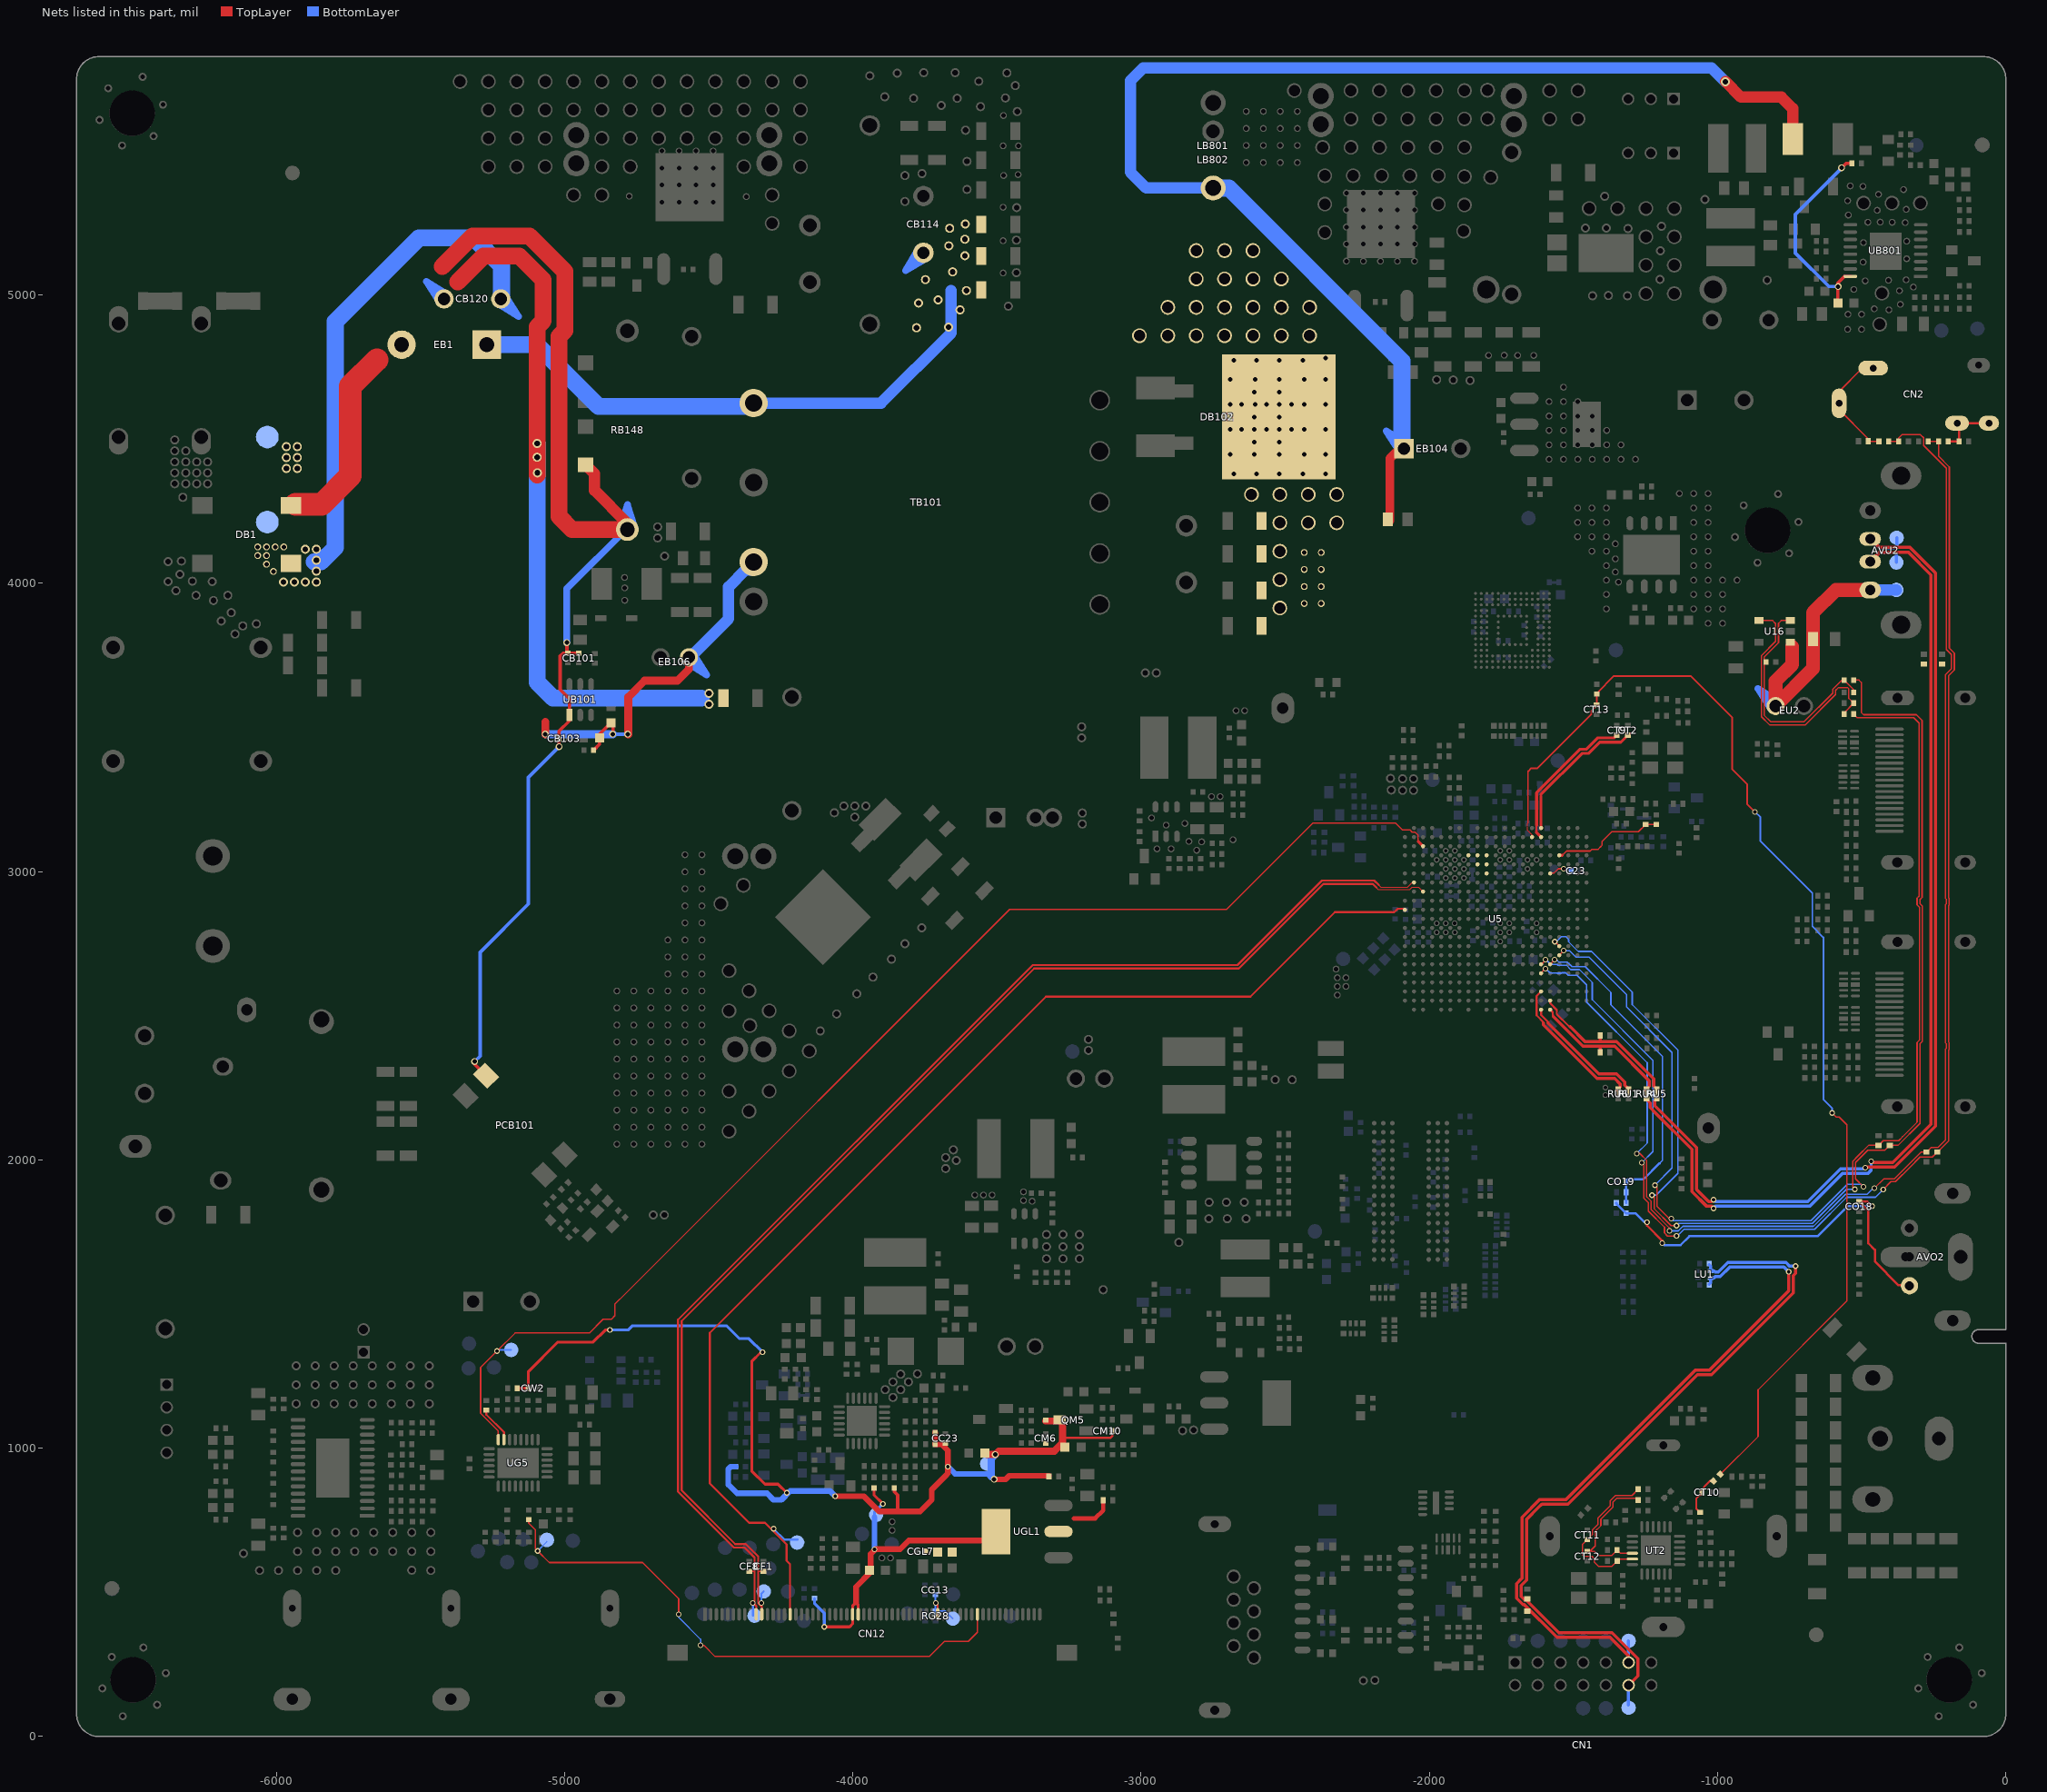
[diagram p0: the nets of this part, all layers, seen from the top]
# Altium PCB MISC84395.PcbDoc (part 23 of 26)
Units mil, origin at the board's own origin, x right, y up, seen from the top; angles counter-clockwise.
Board outline 6692.91 x 5826.77 mil, 2 copper layers (TopLayer, BottomLayer), stack 61.855 mil thick; 951 components, 565 nets, 4374 pads, 1804 vias.
Unrouted connection lines stored in the file: 1.

## Via types
v1: diameter 19.68, hole 11.81, TopLayer to BottomLayer, tented both sides, 1262 vias
v2: diameter 23.62, hole 15.75, TopLayer to BottomLayer, tented both sides, 524 vias
v3: diameter 31.5, hole 19.68, TopLayer to BottomLayer, tented both sides, 11 vias
v4: diameter 24, hole 16, TopLayer to BottomLayer, tented both sides, 6 vias
v5: diameter 19, hole 11.81, TopLayer to BottomLayer, tented both sides, 1 vias

## Nets (pads, with @x,y where several pads share a name; then routed paths per layer and width w, separated by ;. In a path a pad name is that pad's centre, name@x,y a point inside that pad or via, vN(x,y) a via of type N, cw(c..) or ccw(c..) an arc to the next point about the centre after c; other vN are vias at no path point) (continued)
RXO4P/MLV1P: CN12.16 MLV1P.1 U5.M21 | length 4248.8
  TopLayer w3.94: U5.M21@-2088.96,2867.58 U5.M21@-2084.93,2867.58
  TopLayer w7: CN12.16@-4217.44,423.98 -4217.66,424.2 -4217.66,597.66 -4229.66,609.66 -4229.66,666.66 -4304.63,741.63 -4359.87,741.63 -4496,877.76 -4496,1400.29 -3330.29,2566 -2620.46,2566 -2327.36,2859.1 -2236.83,2859.1 -2121.75,2859.1 -2109.53,2871.33 -2088.68,2871.33 U5.M21@-2084.93,2867.58
  BottomLayer w7: v1(-4275,721) -4237,683 MLV1P.1@-4192,683
RXOCN/MLVCKN: CF8.2 CN12.10 MLVCKN.1 U5.R20 | length 4421.4
  TopLayer w3.94: -2175.77,2953.61 -2168.48,2946.32 -2075.73,2946.32 -2059.98,2962.07 U5.R20@-2053.43,2962.07
  TopLayer w7: CF8.2@-4359,573.11 -4340.66,573.11 ; v1(-4347,463) -4344.97,463 v1@-4340.55,458.58 ; CN12.10@-4335.55,423.98 -4334.49,425.05 -4334.49,452.51 v1@-4340.55,458.58 ; -2175.77,2953.61 -2191.26,2969.1 -2372.92,2969.1 -2666.02,2676 -3375.86,2676 -4606,1445.86 -4606,849.17 -4412.46,655.63 -4375.63,655.63 -4340.55,620.55 v1@-4340.55,458.58
  BottomLayer w7: MLVCKN.1@-4346,419 v1@-4346,458
RXOCP/MLVCKP: CF1.2 CN12.11 MLVCKP.1 U5.P19 | length 4443.9
  TopLayer w3.94: -2184.26,2945.13 -2177.58,2938.45 -2067.7,2938.45 -2059.83,2946.32 -2037.68,2946.32 U5.P19@-2021.94,2930.57
  TopLayer w7: -4327.81,573.26 CF1.2@-4310,573.26 ; v1(-4317,463) -4317,452 ; CN12.11@-4315.86,423.98 -4315.86,450.86 -4317,452 ; -2184.26,2945.13 -2196.23,2957.1 -2367.95,2957.1 -2661.05,2664 -3370.89,2664 -4594,1440.89 -4594,854.14 -4407.49,667.63 -4370.66,667.63 -4328.55,625.52 -4328.55,463.55 -4317,452
  BottomLayer w7: v1(-4317,463) -4317,495.5 MLVCKP.1@-4309.04,503.47
SD_CLK_IC: U5.U12
SD_CMD_IC: U5.V12
SD_D0_IC: U5.U13
SD_D1_IC: U5.T12
SD_D2_IC: U5.V13
SD_D3_IC: U5.V14
SET1: RG4.2 UG5.7 | length 127.7
  TopLayer w7: RG4.2@-5271,1132.27 -5271,1116.56 -5210.21,1055.77 UG5.7@-5210.21,1029.71
SGND: CB101.2 CB102.2 CB103.2 CB111.1 CB120.1 DB1.4 DB110.K EB1.2 EB106.2 pad.VIA5@-4499,3580 pad.VIA5@-4499,3618 pad.VIA5@-5094,4383 pad.VIA5@-5095.08,4437 pad.VIA5@-5095.08,4485 pad.VIA5@-5927,4398 pad.VIA5@-5927,4436 pad.VIA5@-5927,4474 pad.VIA5@-5965,4398 pad.VIA5@-5965,4436 pad.VIA5@-5965,4474 PCB101.3 RB103.1 RB104.1 RB130.1 RB148.1 TB101.5 TP-TDT.2 UB101.1 | length 8667.9
  TopLayer w11.81: v2(-5312,2341) -5312,2332 PCB101.3@-5272,2292 ; v2(-5018.49,3433.3) -5018.95,3433.76 CB103.2@-5018.95,3461.3 -5018.95,3486.83 -4982.89,3522.9 UB101.1@-4982.89,3543 -4982.89,3598.7 -5015.49,3631.3 -5015.49,3747.3 -5005.24,3757.55 RB103.1@-4988.43,3757.55 ; v2(-4991.77,3794.3) -4991.77,3760.89 RB103.1@-4988.43,3757.55 ; CB101.2@-4950.43,3757.55 RB103.1@-4988.43,3757.55 ; RB104.1@-4899.02,3421.3 -4878.68,3441.65 CB111.1@-4878.68,3464.3 -4878.68,3476.11 CB102.2@-4838.49,3516.3 -4831.49,3509.3 -4831.49,3477.3 v2(-4832.49,3476.3)
  TopLayer w27.56: v2(-5066.7,3476.3) -5066.7,3518.7 ; v2@-4778.8,3476.3 -4778.8,3605.2 -4722,3662 -4608,3662 -4568.57,3701.43 EB106.2@-4568.57,3743
  TopLayer w39.37: DB110.K@-4927,4410.85 -4896,4379.85 -4896,4322 -4782,4208 RB148.1@-4782,4186.25
  TopLayer w59.06: -5424.5,5098.5 -5319,5204 -5122,5204 -4999,5081 ; -5371,5045 -5281,5135 -5157,5135 -5074,5052 -5074,4910 -5095.08,4888.92 pad.VIA5@-5095.08,4375 ; -5043.89,5126 -4999,5081.11 -4999,5081 ; RB148.1@-4782,4186.25 -4974.25,4186.25 -5019.49,4231.49 -5019.49,4855.51 -4999,4876 -4999,5081
  TopLayer w78.74: DB1.4@-5933.21,4273 -5842.99,4273 -5742.99,4373 -5742.99,4683.01 -5651,4775
  BottomLayer w11.81: v2(-5312,2341) -5293,2360 -5293,2719.57 -5125.22,2887.35 -5125.22,3326.57 v2(-5018.49,3433.3) ; v2(-4832.49,3476.3) v2(-4780.49,3476.3)
  BottomLayer w23.62: v2(-4991.77,3794.3) -4991.77,3981.04 RB148.1@-4782,4190.81
  BottomLayer w27.56: v2(-5066.7,3476.3) v2(-4832.49,3476.3)
  BottomLayer w39.37: EB106.2@-4566.57,3741 -4431,3876.57 -4431,3987.13 -4371.87,4046.26 TB101.5@-4344.32,4046.26
  BottomLayer w59.06: pad.VIA5@-5095.08,4485 -5095.08,3657 -5039.38,3601.3 -4526,3601.3
SPDIF_OUT: AVO2.1 CO18.1 RO4.2 RO45.2 | length 1412
  TopLayer w8: v1(-1245,1784) -1245,1772.56 v1@-1192,1719.56 ; v1@-464.57,1838 -481.56,1855 CO18.1@-508.99,1855 -477.02,1823.03 -477.02,1710.56 -454.72,1688.26 -454.72,1647.72 -372.42,1565.42 AVO2.1@-348.43,1565.42
  BottomLayer w8: RO45.2@-1351.46,1851.06 -1351.46,1848.52 RO4.2@-1318,1815.06 -1284.7,1815.06 v1@-1253.65,1784 ; v1@-1185.29,1704.29 -1129.15,1704.29 -1098.28,1735.16 -653.4,1735.16 -549.12,1839.44 -465.13,1839.44 v1(-464.57,1840)
  other v1: -1192,1711
SPDIF_OUT_IC: CO19.2 DO1.K RO45.1 U5.F5 | length 1153.3
  TopLayer w5: U5.F5@-1580.99,2678.6 v1@-1565.65,2693.95
  BottomLayer w5: v1@-1565.75,2694.33 -1566.45,2695.03 -1559.99,2695.03 -1550.36,2685.4 -1520.83,2685.4 -1505.44,2670.01 -1459.39,2670.01 -1370.3,2580.92 -1370.3,2537.78 -1191.3,2358.78 -1191.3,1998.31 -1201.62,1988
  BottomLayer w8: RO45.1@-1318,1851.06 -1317.07,1851.99 DO1.K@-1317.07,1888 ; DO1.K@-1318,1888.93 CO19.2@-1318,1925.06 -1311.06,1932 -1257.62,1932 -1201.62,1988
  other v1: -1565.49,2694.59
STV: CN12.49 RG81.1 STV.1 | length 1984.8
  TopLayer w5: RG81.1@-5124,752.27 -5124,740 -5101.6,717.6 -5101.6,652.34 v1(-5093.26,644) -5052.76,603.5 -4729.22,603.5 -4604,478.28 v1(-4604,424) ; v1(-4528,316.5) -4516.94,316.5 -4477.94,277.5 -3735.11,277.5 -3682.37,330.24 -3599.58,330.24 -3567.83,361.99 CN12.49@-3567.83,418.08
  BottomLayer w5: v1(-5093.26,644) STV.1@-5061.26,676 ; v1(-4604,424) -4604,413.53 -4528,337.53 v1(-4528,316.5)
STV_IN: STV_IN.1 U5.W19 UG5.8 | length 4440.9
  TopLayer w5: UG5.8@-5229.9,1029.71 -5229.9,1059.9 -5291,1121 -5291,1280 v1(-5234.27,1336.73) -5171.5,1399.5 -4914.01,1399.5 -4866.01,1447.5 -4837.5,1447.5 -4825,1460 -4825,1499.8 -4786.59,1538.21 -3455.8,2869 -2703.54,2869 -2403.72,3168.82 -2118.04,3168.82 -2093.35,3144.14 -2067.15,3144.14 -2059.47,3136.46 -2049.71,3136.46 -2038.85,3125.59 -2038.85,3104.96
  TopLayer w10: -2038.85,3104.96 U5.W19@-2021.94,3088.05
  BottomLayer w5: v1@-5230,1341 STV_IN.1@-5185,1341
SYSTEM_RST_IC: R3.2 R21.1 U5.V4 | length 391.5
  TopLayer w5: U5.V4@-1548.31,3057.74 U5.V4@-1549.5,3056.56 U5.V4@-1546.22,3056.56 ; -1538.63,3057.74 -1537.44,3057.74 -1524.04,3071.14 -1441.86,3071.14 -1435.66,3077.34 -1414.8,3077.34 -1414.76,3077.38 -1414.51,3077.38 -1404.35,3087.54 -1404.35,3087.8 -1401.65,3090.5 -1401.65,3103.21 -1367.01,3137.84 -1274.94,3137.84 R3.2@-1249.77,3163.01 ; R3.2@-1247.5,3160.74 -1245.24,3163.01 R21.1@-1212.77,3163.01
  TopLayer w10: U5.V4@-1549.5,3056.56 -1538.63,3056.56
T-IF-AGC: CT10.2 RT6.2 RT9.1 | length 177.3
  TopLayer w7: RT6.2@-1066.73,777.73 RT6.2@-1061,777.73 -1074.45,791.19 -1074.45,824.61 -1053.89,845.17 CT10.2@-1053.89,847 ; CT10.2@-1054.64,845.25 -1054.64,858.13 ; -1037.77,875 -1054.64,858.13 ; RT9.1@-1014.83,886.17 -1026.6,886.17 -1054.64,858.13
T_SCL: CT12.2 DT3.K RT10.2 UT2.16 | length 488.7
  TopLayer w5: -1405.09,753.36 -1405.09,731.44 ; UT2.16@-1295.78,635.63 -1337.26,635.63 DT3.K@-1348.61,646.98 -1367.52,628.07 -1412.82,628.07 -1426.75,642 -1444,642 -1424.63,661.37 -1424.63,711.9 -1405.09,731.44 ; RT10.2@-1275.74,820 -1282.08,826.34 -1350.18,826.34 -1362.66,813.87 -1362.66,796.49 -1405.09,754.06 -1405.09,731.44
T_SDA: CT11.2 DT2.K RT5.2 UT2.17 | length 548.7
  TopLayer w5: UT2.17@-1295.78,615.94 -1341.46,615.94 DT2.K@-1348.43,608.98 -1366.76,590.65 -1413.4,590.65 -1428,605.25 -1428,617 -1435.89,624.89 -1464.2,624.89 -1469.34,630.04 -1469.34,632.63 -1469.34,665.45 CT11.2@-1452,682.8 -1434.63,700.17 -1434.63,716.04 -1415.09,735.58 -1415.09,758.2 -1372.66,800.63 -1372.66,818.01 -1354.33,836.34 -1297.39,836.34 RT5.2@-1275.74,858
TCON_DVDD: CG12.2 CGL6.1 CGL7.1 CGL49.1 CN12.27 CN12.28 LG02.1 RC6.2 RG24.1 TCON_DVDD.1 UGL1.2 UGL1.4 | length 1358.7
  TopLayer w9: -3989,465.49 -3981.22,457.71 CN12.28@-3981.22,423.98
  TopLayer w10: v1(-4099,380.59) -4011,380.59 -4000.9,390.68 CN12.27@-4000.9,418.08 ; CN12.27@-4000.9,423.98 -4000.9,453.58 -3989,465.49 ; RC6.2@-3926.27,852.18 RC6.2@-3926.27,862 -3926.27,837.27 v1(-3896,807)
  TopLayer w15: -3234,756.5 -3159,756.5 -3131.73,783.77 LG02.1@-3131.73,819
  TopLayer w20: -3989,465.49 -3989,519 CG12.2@-3937.81,570.19 ; CG12.2@-3937.81,577 -3937.81,633.19 v1@-3923.5,647.5 ; v1@-3921.5,649.5 -3836.05,649.5 -3805.55,680 UGL1.4@-3507.54,680
  BottomLayer w10: RG24.1@-4133,479.27 -4133,462 -4099,428 v1(-4099,380.59) ; TCON_DVDD.1@-3925,761 -3925,778 v1(-3896,807)
  BottomLayer w20: v1(-3925,649) -3925,705 TCON_DVDD.1@-3925,761
TP1: CG13.2 CN12.42 RG28.2 RG28.3 TP1.1 | length 168.6
  TopLayer w6: v1(-3712,463) -3705.63,456.63 CN12.42@-3705.63,423.98
  BottomLayer w6: RG28.2@-3714,435.73 -3714,462 CG13.2@-3714,492 ; RG28.2@-3713,434.73 -3678.73,434.73 TP1.1@-3653,409
TUN_AGC_IN_IC: CT13.2 RT7.2 RT9.2 U5.Y7 | length 4147.9
  TopLayer w3.94: -1657.47,3168.35 -1659.73,3166.08 -1659.73,3143.17 -1643.98,3127.42 U5.Y7@-1643.98,3119.55
  TopLayer w5: -1657.47,3168.35 -1657.47,3347.63 ; RT9.2@-990.21,909.83 -859.75,1040.29 -859.75,1202.63 -551.5,1510.88 -551.5,2121.54 -578.88,2148.92 -588.92,2148.92 v1(-603,2163)
  TopLayer w6: -1656.97,3347.63 -1656.97,3348.13 -1646.91,3358.19 -1625.33,3358.19 -1437.49,3546.03 -1437.49,3557.18 -1419.65,3575.03 CT13.2@-1419.65,3578.48 CT13.2@-1419.18,3578.48 ; CT13.2@-1419,3579.13 RT7.2@-1419,3616.27 -1419,3618.85 -1359.83,3678.02 -1093.41,3678.02 -950.15,3534.76 -950.15,3355.62 -897.99,3303.47 -897.99,3234.16 v1(-870.83,3207)
  BottomLayer w6: v1(-870.83,3207) -851.81,3187.97 -851.81,3105.66 -671.46,2925.31 -671.46,2809.93 -633,2771.47 -633,2209.89 -603,2179.89 v1(-603,2163)
TUN_IFM_OUT_IC: CT9.2 U5.Y6 | length 522
  TopLayer w6: -1628.31,3142.32 -1628.31,3159.66
  TopLayer w10: -1628.31,3142.32 -1628.31,3135.15 U5.Y6@-1612.49,3119.32 ; -1628.24,3159.46 -1628.24,3273.26 -1476.75,3424.74 -1454.46,3424.74 -1415.31,3463.9 -1358.76,3463.9 CT9.2@-1349.64,3473
TUN_IFP_OUT_IC: CT2.2 U5.AA6 | length 505.3
  TopLayer w10: U5.AA6@-1613.24,3151.79 -1613.24,3267.04 -1470.54,3409.74 -1448.25,3409.74 -1409.09,3448.9 -1335.76,3448.9 CT2.2@-1311.64,3473 ; U5.AA6@-1612.49,3151.04 U5.AA6@-1612.49,3154 ; U5.AA6@-1611.82,3150.15 U5.AA6@-1611.71,3150.27
UART_RX: CN2.3 CN2.5 DV2.K RV18.1 | length 201.9
  TopLayer w8: RV18.1@-200.1,4492 DV2.K@-162.57,4492 DV2.K@-162.57,4495.62 ; CN2.3@-169.29,4555.12 CN2.5@-59.05,4555.12 ; DV2.K@-162.57,4501 CN2.3@-162.57,4551.55
UART_RX_IC: DV3.K RV17.1 RV18.2 U5.F6 | length 4856.6
  TopLayer w5: U5.F6@-1612.49,2678.6 -1610.87,2678.6 v1@-1595.93,2693.54 ; v1@-1256.16,1983.16 -1256.16,1867.61 -1240.34,1851.79 -1240.34,1822.58 -1184.34,1766.58 -1184.34,1746.55 -1173.92,1736.13 v1(-1142.34,1736.13) ; v1(-426,1897) -398.5,1924.5 -383.09,1924.5 -332.93,1974.66 ; -317.96,1989.63 -332.93,1974.66 ; RV17.1@-269.1,4492 RV18.2@-233.57,4492 -233.57,4440.3 -196.33,4403.07 -196.33,3774.48 -179,3757.14 -179,3698.86 -199.24,3678.62 -199.24,2910.07 -196.49,2907.33 -196.49,2884.67 -199.24,2881.93 -199.24,2409.07 -196.49,2406.33 -196.49,2383.67 -199.24,2380.93 -199.24,2065.49 DV3.K@-238,2026.73 -255.11,2009.63 -297.96,2009.63 -332.93,1974.66
  BottomLayer w4: v1@-1596.03,2695.54 -1579.34,2678.85 -1557.25,2678.85 -1553.53,2675.13
  BottomLayer w5: -1553.26,2675.4 -1524.98,2675.4 -1509.58,2660.01 -1479.4,2660.01 -1434.91,2615.51 -1434.91,2555.71 -1224.3,2345.11 -1224.3,2028.7 v1(-1263,1990) ; v1(-1142.34,1736.13) -1140.2,1736.13 -1116.67,1759.66 -663.55,1759.66 -552.71,1870.5 -452.5,1870.5 v1(-426,1897)
  other v1: -1596.98,2694.59
UART_TX: CN2.2 CN2.4 DV1.K RV16.2 | length 397
  TopLayer w5: DV1.K@-478.14,4494.57 DV1.K@-478.14,4492.68 DV1.K@-477.62,4492.16 ; DV1.K@-478.14,4501.68 -578.74,4602.28 -578.74,4665.26 -497.94,4746.06 CN2.2@-460.63,4746.06 ; DV1.K@-477.62,4492.68 DV1.K@-477.62,4492.16 ; RV16.2@-440.57,4492.16 DV1.K@-477.62,4492.16
UART_TX_IC: DV4.K RV15.1 RV16.1 U5.E6 | length 4939.1
  TopLayer w5: U5.E6@-1612.49,2647.11 -1612.49,2649 v1@-1597.69,2663.8 ; v1(-1280.44,2022.13) -1270.05,2022.13 -1246.16,1998.24 -1246.16,1871.75 -1230.34,1855.94 -1230.34,1826.72 -1167,1763.38 v1(-1167,1753.74) ; v1(-456,1902) -423.5,1934.5 -387.23,1934.5 -295,2026.73 DV4.K@-276,2026.73 -259.64,2043.09 -235.78,2043.09 -209.24,2069.63 -209.24,2385.07 -206.49,2387.82 -206.49,2402.18 -209.24,2404.93 -209.24,2886.07 -206.49,2888.82 -206.49,2903.18 -209.24,2905.93 -209.24,3682.76 -189,3703 ; RV16.1@-407.1,4492.16 RV15.1@-371.57,4492.16 -371.57,4504.27 -360.83,4515 -296.26,4515 -285.46,4504.2 -285.46,4478.05 -206.33,4398.92 -206.33,3770.33 -189,3753 -189,3703 ; -206.33,3685.67 -189,3703
  BottomLayer w4: v1(-1596.98,2663.1) -1581.24,2647.35 -1556.71,2647.35
  BottomLayer w5: -1556.71,2647.35 -1542.77,2647.35 ; -1541.17,2648.94 -1526.81,2648.94 -1517.87,2640.01 -1487.69,2640.01 -1454.91,2607.23 -1454.91,2547.43 -1244.3,2336.82 -1244.3,2058.27 v1(-1280.44,2022.13) ; v1(-1167,1753.74) -1136.74,1753.74 -1120.82,1769.66 -667.69,1769.66 -556.85,1880.5 -481.5,1880.5 -460,1902 v1(-456,1902)
UB801-VCC: CB803.2 RB832.1 UB801.16 | length 722.4
  TopLayer w11.81: CB803.2@-584.86,4972.86 CB803.2@-583,4971 -583,5041 -559.71,5064.29 UB801.16@-539.63,5064.29
  TopLayer w12: v2(-570,5441) -555,5456 RB832.1@-534.73,5456
  BottomLayer w11.81: v2@-584.86,5029 -614.37,5029 -730.72,5145.35 -730.72,5279.28 v2@-570,5440
  other v2: -582,5029
USB2_DM: CN1.11 DM2.1 DU6.K LU1.4 RU2.1 | length 2511.9
  TopLayer w11: -1682.81,545.08 -1697.33,530.57 ; CN1.11@-1309.05,256.74 -1309.06,279.58 -1373.36,343.89 -1557.15,343.89 -1671.17,457.91 -1675.18,457.91 -1697.33,480.06 -1697.33,530.57 ; v1(-753.5,1611.93) -753.5,1545.92 -1027.92,1271.5 -1076.63,1271.5 -1525.63,822.5 -1616.5,822.5 -1679,760 -1679,548.89 -1697.33,530.57
  BottomLayer w11: CN1.11@-1309.05,256.74 DM2.1@-1309,332 ; RU2.1@-1029.27,1569 -1024.35,1573.92 LU1.4@-1024.35,1591.19 -1011.81,1591.19 -1008,1595 -991,1595 -957.5,1628.5 -770.07,1628.5 v1(-753.5,1611.93)
USB2_DM_IC: RU1.2 RU1.3 U5.A6 | length 436.1
  TopLayer w7: U5.A6@-1612.49,2521.12 -1612.49,2502.53 -1586.99,2477.03
  TopLayer w11: -1588.9,2475.11 -1411.79,2298 -1350.21,2298 -1321.83,2269.63 -1321.83,2258.73 RU1.2@-1308.83,2245.73
USB2_DP: CN1.12 DP2.1 DU5.K LU1.1 RU8.1 | length 2627.8
  TopLayer w11: CN1.12@-1309.06,178 -1276.9,210.15 -1276.9,270.06 -1366.74,359.89 -1550.53,359.89 -1664.54,473.91 -1668.55,473.91 -1681.33,486.69 -1681.33,523.94 -1663,542.27 -1663,753.37 -1621.88,794.49 -1609.87,806.5 -1519.01,806.5 -1070.01,1255.5 -1021.29,1255.5 -737.5,1539.29 -737.5,1599.17 -729.84,1606.82 v1(-729.84,1631.52)
  BottomLayer w11: DP2.1@-1309,110 CN1.12@-1309,177.94 ; RU8.1@-1029.27,1637 -1024.35,1632.08 LU1.1@-1024.35,1614.81 -1011.81,1614.81 -1008,1611 -997.63,1611 -964.13,1644.5 -763.44,1644.5 -751.22,1632.28 -730.6,1632.28 v1(-729.84,1631.52)
USB2_DP_IC: RU6.2 RU6.3 U5.C6 | length 504.6
  TopLayer w7: U5.C6@-1612.49,2584.12 -1628.07,2568.53 -1628.07,2501.14 -1603.48,2476.55 -1603.48,2475.14
  TopLayer w11: -1604.9,2475.14 -1604.9,2468.48 -1418.41,2282 -1356.83,2282 -1337.83,2263 -1337.83,2252.73 RU6.2@-1344.83,2245.73
USB3_DM: AVU2.2@-470.76,4074.8 DM3.1 DU3.K RU4.1 | length 3678.3
  TopLayer w11: RU4.1@-1246.83,2210.23 -1234.49,2197.89 -1234.49,2181.37 -1214.28,2161.16 -1214.28,2161.05 -1089.66,2036.43 -1089.66,1890.65 -1038.01,1839 -1021,1839 v1(-1014,1832) ; AVU2.2@-470.76,4074.8 -437.56,4108 -339.46,4108 -260.33,4028.87 -260.33,2123.62 -392.95,1991 -463.04,1991 v1(-467.38,1995.34)
  BottomLayer w11: v1(-1014,1832) -1007,1839 -680.37,1839 -566.93,1952.44 -479.79,1952.44 -467.38,1964.85 v1(-467.38,1995.34) ; AVU2.2@-470.76,4074.8 -438.56,4107 -386,4107 -380,4101 DM3.1@-380,4072
USB3_DM_IC: DU1.K RU4.2 RU4.3 U5.A5 | length 505.9
  TopLayer w7: U5.A5@-1580.99,2521.12 -1571.89,2512.02 -1571.89,2502.06 -1568.47,2498.64
  TopLayer w11: -1569.89,2497.23 -1467.07,2394.41 -1357.5,2394.41 -1236.83,2273.75 -1236.83,2255.73 RU4.2@-1246.83,2245.73 ; DU1.K@-1407.25,2372.74 -1407.25,2393.15
USB3_DP: AVU2.3 DP3.1 DU4.K RU5.1 | length 3678.6
  TopLayer w11: RU5.1@-1214,2209 -1218.49,2204.51 -1218.49,2188 -1198.28,2167.79 ; RU5.1@-1211.77,2210.23 RU5.1@-1210.83,2210.23 ; -1198.28,2167.68 -1073.66,2043.05 -1073.66,1897.28 -1048.46,1872.08 ; -1063.69,1887.31 -1048.46,1872.08 ; v1@-1016,1864 v1(-1014,1862) -1021,1855 -1031.38,1855 -1048.46,1872.08 ; v1(-488,1973) -486,1975 -386.33,1975 -244.33,2116.99 -244.33,4035.5 -332.84,4124 -437.84,4124 AVU2.3@-469.07,4155.23
  BottomLayer w11: v1(-1014,1862) -1007,1855 -687,1855 -573.56,1968.44 -531,1968.44 v1@-495.56,1968.44 ; AVU2.3@-470.76,4153.54 -440.22,4123 -386,4123 -379,4130 DP3.1@-379,4158
USB3_DP_IC: DU2.K RU5.2 RU5.3 U5.B5 | length 545.8
  TopLayer w7: U5.B5@-1580.99,2552.62 -1580.99,2543.17 -1557.59,2519.76 -1557.59,2504.73 -1513.41,2460.55
  TopLayer w11: -1511.92,2462.03 -1460.3,2410.41 -1350.87,2410.41 -1220.83,2280.38 -1220.83,2255.73 RU5.2@-1210.83,2245.73 ; -1407.25,2411.15 DU2.K@-1407.25,2431.74
USB_5V: AVU2.1@-470.76,3976.38 CU1.2 EU2.1 U16.1 USB_5V.1 | length 929.1
  TopLayer w48: -742,3780 -742,3718 -799.05,3660.95 EU2.1@-799.05,3574 -668.87,3704.18 CU1.2@-668.87,3806 -668.87,3897.97 -590.46,3976.38 AVU2.1@-470.76,3976.38
  BottomLayer w40: AVU2.1@-470.76,3976.38 -470.14,3977 USB_5V.1@-380,3977
USB_EN: RU9.1 RU12.2 U16.4 | length 891.7
  TopLayer w5: U16.4@-855.97,3870.4 -809.24,3870.4 -798.83,3860 -798.83,3798.17 -848.09,3748.91 -848.09,3549.05 -848.04,3549 -848.04,3537.07 -820.15,3509.17 -695.47,3509.17 -590.74,3613.91 -590.74,3628.1 -580.49,3638.34 -549.6,3638.34 -544.83,3633.57 -544.83,3600.73 RU9.1@-528.1,3584 -561.57,3550.54 RU12.2@-561.57,3546
USB_EN_IC: DU9.K RU12.1 U5.H4 | length 4017.5
  TopLayer w5: v1@-1564.9,2757 U5.H4@-1549.5,2741.6 ; -1220.34,1870.46 -1220.34,1830.86 -1161.48,1772 v1(-1143,1772) ; RU12.1@-528.1,3546 -516.1,3534 -320.33,3534 -301.03,3514.69 -301.03,2914.64 -308.34,2907.33 -308.34,2884.67 -300.03,2876.36 -300.03,2415.35 -308.33,2407.04 -308.33,2130.67 -358.71,2080.29 -372.37,2066.63 -425.64,2066.63 DU9.K@-442,2050.27 -476.51,2050.27 -512.48,2014.3 -531.5,1995.28 -531.5,1905.5 v1(-524,1898)
  BottomLayer w5: v1@-1559.24,2756.86 -1541.41,2774.69 -1527.05,2774.69 -1516.89,2764.53 -1516.89,2756.41 -1483.49,2723.01 -1437.43,2723.01 -1296.3,2581.88 -1296.3,2538.73 -1138.3,2380.73 -1138.3,1953.31 -1213.8,1877.8 v1(-1227.69,1877.8) ; v1(-1143,1772) -1135.34,1779.66 -671.83,1779.66 -553.49,1898 v1(-524,1898)
  other v1: -1565.24,2756.86
USB_FLT: RU3.1 RU7.2 RU10.2 U16.3 | length 795.4
  TopLayer w5: U16.3@-747.7,3870.4 -779.43,3870.4 -788.83,3861 -788.83,3794.02 -838.04,3744.81 -838.04,3541.21 -816.01,3519.17 -700.3,3519.17 -600.74,3618.74 -600.74,3632.24 -568.98,3664 RU7.2@-561.57,3664 ; RU7.2@-561.12,3664 -528.1,3630.98 RU3.1@-528.1,3621
USB_FLT_IC: DU8.K RU7.1 U5.G4 | length 4053.9
  TopLayer w5: U5.G4@-1549.5,2710.1 v1@-1534.59,2725 ; v1(-1217.69,1912.59) -1210.34,1905.25 -1210.34,1838.82 -1167.68,1796.15 v1(-1161.11,1796.15) ; RU7.1@-528.1,3664 -509.83,3664 -501.83,3656 -501.83,3552 -493.83,3544 -310.33,3544 -291.03,3524.69 -291.03,2910.5 -298.34,2903.18 -298.34,2888.82 -290.03,2880.5 -290.03,2411.21 -298.33,2402.9 -298.33,2126.52 -374.59,2050.27 DU8.K@-403,2050.27 -419.77,2033.5 -479.13,2033.5 -521.5,1991.13 -521.5,1934.5 v1(-494,1907)
  BottomLayer w5: v1(-1534.23,2725.85) -1514.61,2725.85 -1491.77,2703.01 -1445.72,2703.01 -1316.3,2573.59 -1316.3,2530.45 -1158.3,2372.45 -1158.3,1971.97 v1(-1217.69,1912.59) ; v1@-1156.96,1792 v1@-1154.61,1792 ; v1@-1154.61,1789.66 -675.97,1789.66 -550.29,1915.34 -502.34,1915.34 v1(-494,1907)
VBL: DB102.2 DB802.K EB104.1@-2087.9,4467 LB801.1@-2750.11,5370.72 LB802.1 pad.VIA5@-973,5739 pad.VIA5@-2321.68,4209.41 pad.VIA5@-2321.68,4307.83 pad.VIA5@-2375.01,3929.43 pad.VIA5@-2375.01,3988.48 pad.VIA5@-2375.01,4047.54 pad.VIA5@-2375.01,4106.59 pad.VIA5@-2415.25,4858.41 pad.VIA5@-2415.25,4956.83 pad.VIA5@-2420.1,4209.41 pad.VIA5@-2420.1,4307.83 pad.VIA5@-2434.06,3929.43 pad.VIA5@-2434.06,3988.48 pad.VIA5@-2434.06,4047.54 pad.VIA5@-2434.06,4106.59 pad.VIA5@-2513.68,4858.41 pad.VIA5@-2513.68,4956.83 pad.VIA5@-2513.68,5055.26 pad.VIA5@-2518.53,3914.13 pad.VIA5@-2518.53,4012.56 pad.VIA5@-2518.53,4110.98 pad.VIA5@-2518.53,4209.41 pad.VIA5@-2518.53,4307.83 pad.VIA5@-2612.1,4858.41 pad.VIA5@-2612.1,4956.83 pad.VIA5@-2612.1,5055.26 pad.VIA5@-2612.1,5153.68 pad.VIA5@-2616.95,4307.83 pad.VIA5@-2710.53,4858.41 pad.VIA5@-2710.53,4956.83 pad.VIA5@-2710.53,5055.26 pad.VIA5@-2710.53,5153.68 pad.VIA5@-2808.95,4858.41 pad.VIA5@-2808.95,4956.83 pad.VIA5@-2808.95,5055.26 pad.VIA5@-2808.95,5153.68 pad.VIA5@-2907.38,4858.41 pad.VIA5@-2907.38,4956.83 pad.VIA5@-3005.8,4858.41 RB124.2 RB125.2 RB126.2 RB136.2 RB140.1 | length 4554.4
  TopLayer w31.5: RB140.1@-2137,4217 -2137,4432.43 EB104.1@-2092.43,4477
  TopLayer w39.37: pad.VIA5@-973,5740 -919,5686 -779,5686 -739.61,5646.61 DB802.K@-739.61,5541
  BottomLayer w39.37: LB801.1@-2750.11,5370.72 -2981.72,5370.72 -3037.11,5426.11 -3037.11,5742.59 -2993.11,5786.59 -1020.59,5786.59 pad.VIA5@-973,5739
  BottomLayer w59.06: LB801.1@-2750.11,5370.72 -2695.72,5370.72 -2095.43,4770.43 -2095.43,4504
  other v2: -2678.7,4379.7 -2599.96,4379.7 -2521.22,4379.7 -2438.54,4379.7 -2359.8,4379.7 -2690.51,4446.63 -2607.83,4446.63 -2521.22,4446.63 -2434.61,4446.63 -2359.8,4446.63 -2607.83,4489.94 -2521.22,4489.94 -2690.51,4533.24 -2651.14,4533.24 -2607.83,4533.24 -2564.53,4533.24 -2521.22,4533.24 -2477.91,4533.24 -2434.61,4533.24 -2359.8,4533.24 -2607.83,4576.55 -2521.22,4576.55 -2690.51,4619.86 -2651.14,4619.86 -2603.9,4619.86 -2564.53,4619.86 -2521.22,4619.86 -2477.91,4619.86 -2434.61,4619.86 -2359.8,4619.86 -2607.83,4663.16 -2521.22,4663.17 -2690.51,4706.47 -2603.9,4706.47 -2521.22,4706.47 -2434.61,4706.47 -2359.8,4706.47 -2678.7,4773.4 -2599.96,4773.4 -2521.22,4773.4 -2438.54,4773.4 -2359.8,4781.28
VBRIDGE: CB114.2 CB120.2 DB1.1 EB1.1@-5269.73,4827.43 pad.VIA5@-3606,5015 pad.VIA5@-3610,5246 pad.VIA5@-3611,5136 pad.VIA5@-3611,5193 pad.VIA5@-3628,4948 pad.VIA5@-3654,5080 pad.VIA5@-3664,5231 pad.VIA5@-3667,5170 pad.VIA5@-3668,4888 pad.VIA5@-3704,4983 pad.VIA5@-3748,5053 pad.VIA5@-3772,4972 pad.VIA5@-3779,4886 pad.VIA5@-5861,4004 pad.VIA5@-5861,4042 pad.VIA5@-5861,4080 pad.VIA5@-5861,4118 pad.VIA5@-5899,4004 pad.VIA5@-5899,4118 pad.VIA5@-5937,4004 pad.VIA5@-5974,4126 pad.VIA5@-5975,4004 pad.VIA5@-6004,4126 pad.VIA5@-6010,4041 pad.VIA5@-6034,4066 pad.VIA5@-6034,4096 pad.VIA5@-6034,4126 pad.VIA5@-6064,4096 pad.VIA5@-6064,4126 RB152.2 RB153.2 RB156.2 TB101.1 TP-TDT.1 | length 3634.7
  BottomLayer w39.37: TB101.1@-4318.02,4623.74 -3903,4623.74 ; -3902.56,4624.56 -3659.11,4868 -3659.11,5015.52
  BottomLayer w59.06: pad.VIA5@-5869,4074 -5845,4074 -5795,4124 -5795,4908 -5505,5198 -5316,5198 -5218.57,5100.57 CB120.2@-5218.57,4987 ; EB1.1@-5269.73,4827.43 -5096.43,4827.43 -4881.96,4612.96 TB101.1@-4359.83,4612.96
VCC_PANEL_IN: CC23.2 CM6.2 CM7.2 CM9.2 CM10.1 CW2.1 QM5.D RC10.2 RC14.2 RC15.2 RC20.1 RG01.2 RM3.1 RW1.1 VCC_PANEL.1 | length 3859.8
  TopLayer w8: -3271.51,1035.51 -3106.49,1035.51 -3100.27,1041.73 CM10.1@-3100.27,1060
  TopLayer w10: RW1.1@-5164.27,1208 CW2.1@-5125.89,1208 -5125.89,1265.11 -5023,1368 -4900.96,1368 -4858.96,1410 v1(-4843,1410) ; v1(-4313.5,1333) -4318.7,1333 -4350.5,1301.2 -4350.5,921.06 -4304.57,875.13 -4265.37,875.13 -4259.13,875.13 v1(-4229,845)
  TopLayer w12: RC10.2@-3856.27,862 -3856.27,849.74 -3844.16,837.63 -3844.16,782.59
  TopLayer w20: v1(-4061,833.59) -3961.96,833.59 -3909.12,780.75 -3766.84,780.75 -3726,821.58 -3726,857.07 -3675.53,907.53 ; RC15.2@-3714.27,1054 RC14.2@-3714.27,1014 -3692.09,1014 ; CC23.2@-3687.04,1008.96 -3670.4,992.32 v1(-3670.4,936) -3670.4,912.66 ; v2(-3510,892) -3470.03,892 -3457.42,904.61 RG01.2@-3319.73,904.61
  TopLayer w25: CM9.2@-3542.19,984 -3536.19,978 v2(-3506,978) -3493.84,990.16 -3300.84,990.16 -3273,1018 -3273,1088.72 -3278.65,1094.37 RM3.1@-3331,1094.37
  BottomLayer w10: v1(-4843,1410) -4779.5,1410 -4765.5,1424 -4436.89,1424 -4392.89,1380 -4360.2,1380 -4313.5,1333.3 v1(-4313.5,1333)
  BottomLayer w20: RC20.1@-4405.73,936.19 -4423.81,936.19 -4432,928 -4432,874.13 -4401.81,843.94 -4297.82,843.94 -4275.01,821.13 -4247.87,821.13 -4217,852 -4079.41,852 v1(-4061,833.59) ; v1(-3670.4,936) -3645.4,911 -3534.42,911 -3532.61,909.18
  BottomLayer w25: -3520,902 -3520,964 v2(-3506,978)
VCOM_IN_IC: C23.1 U5.T5 | length 82.3
  TopLayer w5: U5.T5@-1580.99,2993.56 -1579.27,2995.29 -1566.99,2995.29 -1552.43,3009.84 v1@-1534.56,3009.84
  BottomLayer w5: v1@-1534.56,3009.84 -1515.48,3009.84 C23.1@-1508.37,3002.74
  other v1: -1533.99,3009.55